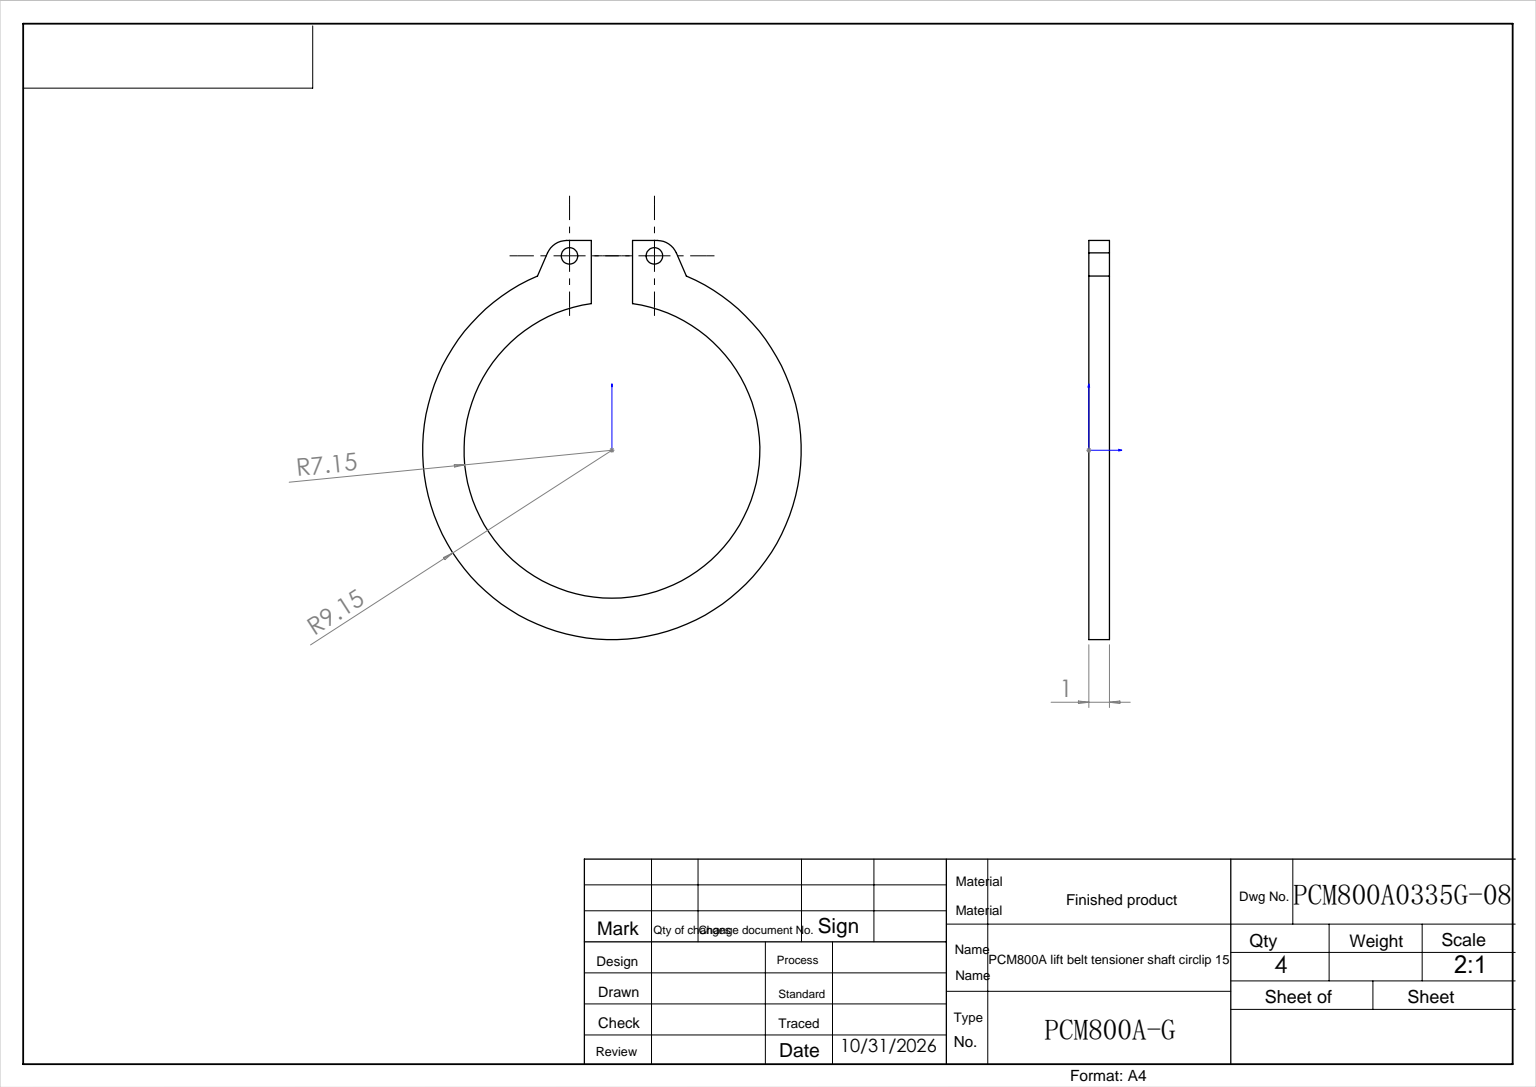
SolidWorks part; units mm, degrees
ref_plane "前视" through (0, 0, 0) normal (0, 0, 1) x (1, 0, 0)
ref_plane "上视" through (0, 0, 0) normal (0, 1, 0) x (1, 0, 0)
ref_plane "右视" through (0, 0, 0) normal (1, 0, 0) x (0, 0, -1)
sketch "草图1" plane through (0, 0, 0) normal (1, 0, 0) x (0, 0, -1)
  circle A0 centre (0, 0) radius 7.15
  circle A1 centre (0, 0) radius 9.15
extrude "拉伸1" add sketch "草图1" along normal blind 1
sketch "草图2" plane through (1, 0, 0) normal (1, 0, 0) x (0, 0, -1)
  line L1 (-1, 0) -> (1, 0)
  line L2 (-1, 0) -> (-1, 11.5616)
  line L3 (-1, 11.5616) -> (1, 11.5616)
  line L4 (1, 0) -> (1, 11.5616)
  dimension "D1" = 2
  dimension "D2" = 1
extrude "切除-拉伸1" cut sketch "草图2" against normal through all
sketch "草图3" plane through (1, 0, 0) normal (1, 0, 0) x (0, 0, -1)
  line L0 (-1, 9.0952) -> (-1, 10.1255)
  line L1 (-1, 10.1255) -> (-2.197, 10.1255)
  line L2 (-3.1135, 9.5257) -> (-3.5997, 8.4122)
  line L3 (0, 0) -> (0, 8.3037) construction
  line L4 (1, 9.0952) -> (1, 10.1255)
  line L5 (3.1135, 9.5257) -> (3.5997, 8.4122)
  line L6 (1, 10.1255) -> (2.197, 10.1255)
  circle A0 centre (0, 0) radius 9.15 construction
  arc A1 (-3.1135, 9.5257) -> (-2.197, 10.1255) centre (-2.197, 9.1255) cw
  arc A2 (3.5997, 8.4122) -> (1, 9.0952) centre (0, 0) ccw
  arc A3 (3.1135, 9.5257) -> (2.197, 10.1255) centre (2.197, 9.1255) ccw
  arc A4 (-1, 9.0952) -> (-3.5997, 8.4122) centre (0, 0) ccw
  circle A5 centre (-2.0521, 9.3832) radius 0.4
  circle A6 centre (2.0521, 9.3832) radius 0.4
  dimension "D1" = 1
extrude "拉伸2" add sketch "草图3" against normal blind 1
